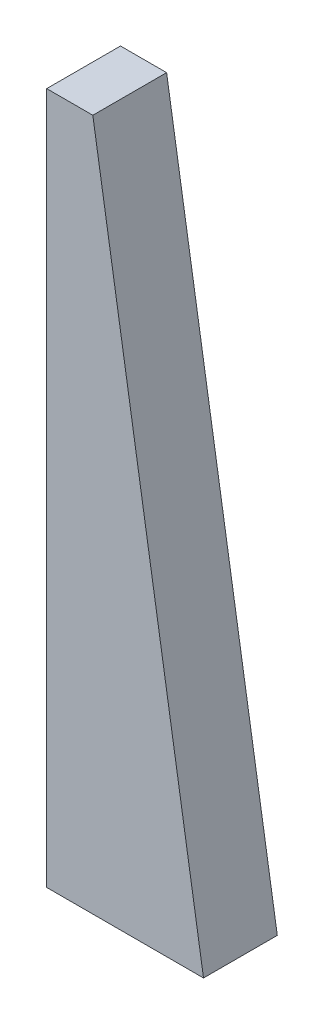
SolidWorks part; units mm, degrees
material "普通碳钢"
ref_plane "Front Plane" through (0, 0, 0) normal (0, 0, 1) x (1, 0, 0)
ref_plane "Top Plane" through (0, 0, 0) normal (0, 1, 0) x (1, 0, 0)
ref_plane "Right Plane" through (0, 0, 0) normal (1, 0, 0) x (0, 0, -1)
sketch "Sketch1" plane through (0, 0, 0) normal (0, 0, 1) x (1, 0, 0)
  line L0 (0, 0) -> (34, 0)
  line L1 (0, 0) -> (0, 150)
  line L2 (0, 150) -> (10, 150)
  line L3 (10, 150) -> (34, 0)
  dimension "D1" = 34
  dimension "D2" = 150
  dimension "D3" = 10
extrude "Extrude1" add sketch "Sketch1" along normal mid plane 16
